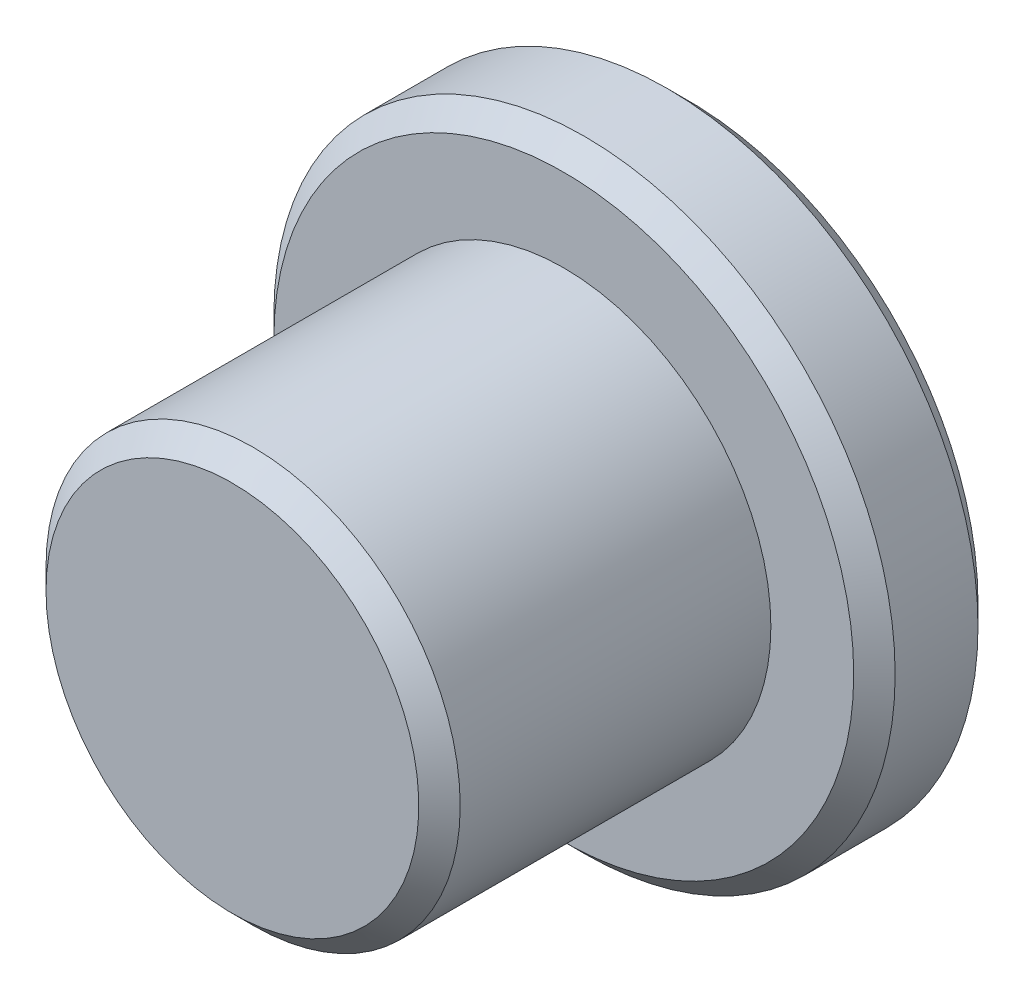
from build123d import *

# Parameters (mm, degrees)
CHAMFER1_SIZE = 0.5


with BuildPart() as part:
    # Sketch1 → Revolve1 (revolve)
    with BuildSketch(Plane(origin=(0, 0, 0), x_dir=(0, 0, -1), z_dir=(1, 0, 0)), mode=Mode.PRIVATE) as revolve1_sk:
        Polygon((11, 0), (11, 7.5), (8, 7.5), (8, 5), (0, 5), (0, 0), align=None)
    revolve(revolve1_sk.sketch.rotate(Axis((0, 0, 0), (0, 0, -1)), 90), axis=Axis((0, 0, 0), (0, 0, -1)))

    # Chamfer1
    chamfer1_edges = [part.edges().sort_by_distance(p)[0] for p in [
        (-5, 0, 0),
        (-7.5, 0, -8),
        (-7.5, 0, -11),
    ]]
    chamfer(chamfer1_edges, length=CHAMFER1_SIZE)


solid = part.part
